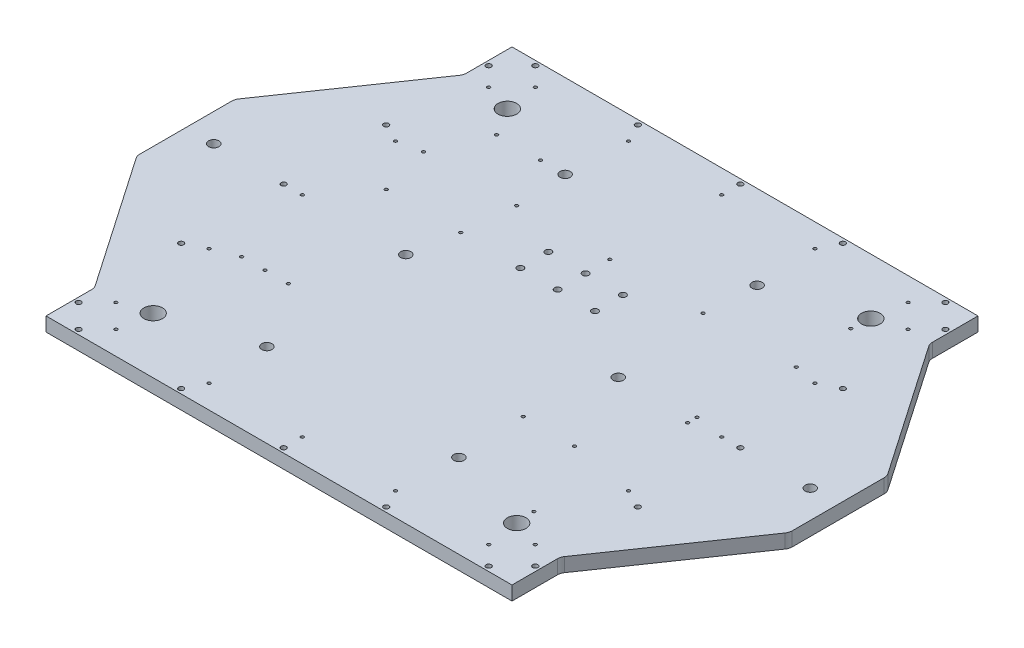
SolidWorks part; units mm, degrees
material "6061Al"
ref_plane "前视基准面" through (0, 0, 0) normal (0, 0, 1) x (1, 0, 0)
ref_plane "上视基准面" through (0, 0, 0) normal (0, 1, 0) x (1, 0, 0)
ref_plane "右视基准面" through (0, 0, 0) normal (1, 0, 0) x (0, 0, -1)
sketch "草图1" plane through (0, 0, 0) normal (0, 1, 0) x (1, 0, 0)
  line L1 (-350, -250) -> (350, -250)
  line L2 (-350, -250) -> (-350, 250)
  line L3 (-350, 250) -> (350, 250)
  line L4 (350, -250) -> (350, 250)
  line L5 (-350, -250) -> (350, 250) construction
  line L6 (-350, 250) -> (350, -250) construction
  point P0 (0, 0)
  dimension "D1" = 700
  dimension "D2" = 500
extrude "凸台-拉伸1" add sketch "草图1" along normal blind 15
sketch "草图2" plane through (0, 15, 0) normal (0, 1, 0) x (1, 0, 0)
  line L0 (-250, 250) -> (-250, 198)
  line L1 (350, 250) -> (-350, 250) construction
  line L2 (-250, 198) -> (-350, 52.5)
  line L3 (-350, 250) -> (-350, 52.5)
  line L4 (-350, 250) -> (-350, -250) construction
  line L5 (-350, 0) -> (0, 0) construction
  line L6 (0, 0) -> (0, 250) construction
  line L7 (-350, 250) -> (-250, 250)
  line L8 (350, 250) -> (250, 250)
  line L9 (350, 250) -> (350, 52.5)
  line L10 (250, 198) -> (350, 52.5)
  line L11 (250, 250) -> (250, 198)
  line L12 (250, -250) -> (250, -198)
  line L13 (250, -198) -> (350, -52.5)
  line L14 (350, -250) -> (350, -52.5)
  line L15 (350, -250) -> (250, -250)
  line L16 (-350, -250) -> (-250, -250)
  line L17 (-350, -250) -> (-350, -52.5)
  line L18 (-250, -198) -> (-350, -52.5)
  line L19 (-250, -250) -> (-250, -198)
  dimension "D1" = 52
  dimension "D2" = 100
  dimension "D3" = 105
extrude "切除-拉伸1" cut sketch "草图2" against normal through all
hole_wizard "M5 六角凹头螺钉的柱形沉头孔2" positions "草图3" profile "草图4" counterbore size "M5" standard "ISO" end condition through all
sketch "草图3" plane through (0, 0, 0) normal (0, -1, 0) x (-1, 0, 0)
  line L0 (0, 0) -> (0, 372.2873) construction
  line L2 (0, 0) -> (463.0821, 0) construction
  point P0 (-220, 245)
  point P3 (-110, 245)
  point P6 (-110, 245)
  point P8 (0, 245)
  point P11 (110, 245)
  point P14 (220, 245)
  point P17 (245, 220)
  point P20 (245, 110)
  point P33 (245, 0)
  point P37 (245, -110)
  point P38 (245, -220)
  point P39 (220, -245)
  point P40 (110, -245)
  point P41 (0, -245)
  point P42 (-110, -245)
  point P43 (-220, -245)
  point P44 (-245, -220)
  point P45 (-245, -110)
  point P46 (-245, 0)
  point P47 (-245, 110)
  point P48 (-245, 220)
sketch "草图4" plane through (220, 0, -245) normal (1, 0, 0) x (0, 0, -1)
  line L0 (0, 0) -> (0, 15)
  line L1 (0, 15) -> (2.75, 15)
  line L3 (2.75, 15) -> (2.75, 5.4)
  line L4 (2.75, 5.4) -> (4.95, 5.4)
  line L5 (4.95, 5.4) -> (4.95, 0)
  line L7 (4.95, 0) -> (0, 0)
  line L11 (0, -6.35) -> (0, 107.95) construction
  dimension "通孔孔直径" = 5.5
  dimension "通孔孔深度" = 15
  dimension "柱形沉头孔直径" = 9.9
  dimension "柱形沉头孔深度" = 5.4
hole_wizard "M10 间隙孔1" positions "草图5" profile "草图6" hole size "M10" standard "ISO" end condition through all
sketch "草图5" plane through (0, 0, 0) normal (0, -1, 0) x (-1, 0, 0)
  line L0 (0, 0) -> (0, 300.0763) construction
  line L2 (-350, -52.5) -> (-350, 52.5) construction
  line L3 (0, 0) -> (425.5875, 0) construction
  point P0 (-320, 0)
  point P2 (-114, 0)
  point P13 (114, 0)
  point P14 (320, 0)
  point P15 (-103, 160)
  point P18 (103, 160)
  point P27 (103, -160)
  point P28 (-103, -160)
  dimension "D1" = 206
  dimension "D2" = 30
sketch "草图6" plane through (320, 0, 0) normal (1, 0, 0) x (0, 0, -1)
  line L0 (0, 0) -> (0, 15)
  line L1 (0, 15) -> (5.5, 15)
  line L2 (5.5, 15) -> (5.5, 0)
  line L5 (5.5, 0) -> (0, 0)
  line L11 (0, -6.35) -> (0, 107.95) construction
  dimension "通孔孔直径" = 11
  dimension "通孔孔深度" = 15
sketch "草图9" plane through (0, 0, 0) normal (0, -1, 0) x (1, 0, 0)
  line L1 (-195, 190) -> (195, 190) construction
  line L2 (-195, 190) -> (-195, -190) construction
  line L3 (-195, -190) -> (195, -190) construction
  line L4 (195, 190) -> (195, -190) construction
  line L5 (-195, 190) -> (195, -190) construction
  line L6 (-195, -190) -> (195, 190) construction
  circle A1 centre (195, 190) radius 10
  circle A2 centre (195, -190) radius 10
  circle A3 centre (-195, -190) radius 10
  circle A4 centre (-195, 190) radius 10
  point P0 (0, 0)
  dimension "D1" = 20
  dimension "D2" = 380
  dimension "D3" = 390
extrude "切除-拉伸2" cut sketch "草图9" against normal through all
hole_wizard "M8 螺纹孔2" positions "草图10" profile "草图11" tap size "M8" standard "ISO" end condition up to next
sketch "草图10" plane through (0, 15, 0) normal (0, 1, 0) x (1, 0, 0)
  point P0 (-40, 79)
  point P3 (0, 79)
  point P6 (40, 79)
  point P9 (40, 49)
  point P12 (0, 49)
  point P15 (-40, 49)
sketch "草图11" plane through (-40, 15, -79) normal (1, 0, 0) x (0, 0, 1)
  line L0 (0, 0) -> (0, 15)
  line L1 (0, 15) -> (3.4, 15)
  line L2 (3.4, 15) -> (3.4, 0)
  line L5 (3.4, 0) -> (0, 0)
  line L11 (0, -6.35) -> (0, 107.95) construction
  dimension "通孔螺纹孔钻头直径" = 6.8
  dimension "通孔螺纹孔钻头深度" = 15
cosmetic thread "孔螺蚊线7" parameters "D2"=8
cosmetic thread "孔螺蚊线8" parameters "D2"=8
cosmetic thread "孔螺蚊线9" parameters "D2"=8
cosmetic thread "孔螺蚊线10" parameters "D2"=8
cosmetic thread "孔螺蚊线11" parameters "D2"=8
cosmetic thread "孔螺蚊线12" parameters "D2"=8
hole_wizard "M4 螺纹孔1" positions "草图12" profile "草图13" tap size "M4" standard "ISO" end condition through all
sketch "草图12" plane through (0, 15, 0) normal (0, 1, 0) x (1, 0, 0)
  line L0 (0, 250) -> (0, 0) construction
  line L1 (250, 250) -> (-250, 250) construction
  line L3 (0, 225) -> (100, 225) construction
  line L4 (0, 0) -> (381.3824, 0) construction
  line L5 (250, -198) -> (250, -250) construction
  line L6 (225, 0) -> (225, 100) construction
  line L7 (-225, 0) -> (-225, 100) construction
  line L8 (0, -225) -> (100, -225) construction
  line L9 (0, 105) -> (100, 105) construction
  line L10 (-100, 225) -> (-100, 105) construction
  point P0 (0, 225)
  point P12 (100, 225)
  point P13 (200, 225)
  point P16 (-200, 225)
  point P17 (-100, 225)
  point P23 (225, 0)
  point P32 (225, 100)
  point P33 (225, 200)
  point P36 (225, -200)
  point P37 (225, -100)
  point P40 (-225, -100)
  point P41 (-225, -200)
  point P42 (-225, 200)
  point P43 (-225, 100)
  point P44 (-225, 0)
  point P47 (-100, -225)
  point P48 (-200, -225)
  point P49 (200, -225)
  point P50 (100, -225)
  point P51 (0, -225)
  point P56 (0, 105)
  point P57 (100, 105)
  point P58 (200, 105)
  point P61 (-200, 105)
  point P62 (-100, 105)
  dimension "D1" = 25
  dimension "D3" = 100
  dimension "D4" = 25
  dimension "D6" = 100
  dimension "D8" = 120
  dimension "D2" = 3
  dimension "D5" = 3
  dimension "D7" = 2
sketch "草图13" plane through (0, 15, -225) normal (1, 0, 0) x (0, 0, 1)
  line L0 (0, 0) -> (0, 15)
  line L1 (0, 15) -> (1.65, 15)
  line L2 (1.65, 15) -> (1.65, 0)
  line L5 (1.65, 0) -> (0, 0)
  line L11 (0, -6.35) -> (0, 107.95) construction
  dimension "通孔螺纹孔钻头直径" = 3.3
  dimension "通孔螺纹孔钻头深度" = 15
cosmetic thread "孔螺蚊线13" parameters "D2"=4
cosmetic thread "孔螺蚊线14" parameters "D2"=4
cosmetic thread "孔螺蚊线15" parameters "D2"=4
cosmetic thread "孔螺蚊线16" parameters "D2"=4
cosmetic thread "孔螺蚊线17" parameters "D2"=4
cosmetic thread "孔螺蚊线18" parameters "D2"=4
cosmetic thread "孔螺蚊线19" parameters "D2"=4
cosmetic thread "孔螺蚊线20" parameters "D2"=4
cosmetic thread "孔螺蚊线21" parameters "D2"=4
cosmetic thread "孔螺蚊线22" parameters "D2"=4
cosmetic thread "孔螺蚊线23" parameters "D2"=4
cosmetic thread "孔螺蚊线24" parameters "D2"=4
cosmetic thread "孔螺蚊线25" parameters "D2"=4
cosmetic thread "孔螺蚊线26" parameters "D2"=4
cosmetic thread "孔螺蚊线27" parameters "D2"=4
cosmetic thread "孔螺蚊线28" parameters "D2"=4
cosmetic thread "孔螺蚊线29" parameters "D2"=4
cosmetic thread "孔螺蚊线30" parameters "D2"=4
cosmetic thread "孔螺蚊线31" parameters "D2"=4
cosmetic thread "孔螺蚊线32" parameters "D2"=4
cosmetic thread "孔螺蚊线46" parameters "D2"=4
cosmetic thread "孔螺蚊线47" parameters "D2"=4
cosmetic thread "孔螺蚊线48" parameters "D2"=4
cosmetic thread "孔螺蚊线49" parameters "D2"=4
cosmetic thread "孔螺蚊线50" parameters "D2"=4
hole_wizard "M4 螺纹孔2" positions "草图14" profile "草图15" tap size "M4" standard "ISO" end condition through all
sketch "草图14" plane through (0, 15, 0) normal (0, 1, 0) x (1, 0, 0)
  line L0 (-350, 52.5) -> (-350, -52.5) construction
  point P0 (-185, 50)
  point P3 (-105, 50)
  point P6 (-176.5, 160)
  point P9 (-129.5, 160)
  point P12 (193.5, 170)
  point P15 (193.5, 5)
  point P18 (193.5, -5)
  point P21 (193.5, -170)
  point P24 (99.5, -87.5)
  point P27 (154.5, -87.5)
  point P31 (-150, -90)
  point P33 (-200, -90)
  point P36 (-175, -90)
  dimension "D1" = 50
  dimension "D2" = 25
  dimension "D3" = 150
  dimension "D4" = 90
sketch "草图15" plane through (-185, 15, -50) normal (1, 0, 0) x (0, 0, 1)
  line L0 (0, 0) -> (0, 15)
  line L1 (0, 15) -> (1.65, 15)
  line L2 (1.65, 15) -> (1.65, 0)
  line L5 (1.65, 0) -> (0, 0)
  line L11 (0, -6.35) -> (0, 107.95) construction
  dimension "通孔螺纹孔钻头直径" = 3.3
  dimension "通孔螺纹孔钻头深度" = 15
cosmetic thread "孔螺蚊线33" parameters "D2"=4
cosmetic thread "孔螺蚊线34" parameters "D2"=4
cosmetic thread "孔螺蚊线35" parameters "D2"=4
cosmetic thread "孔螺蚊线36" parameters "D2"=4
cosmetic thread "孔螺蚊线37" parameters "D2"=4
cosmetic thread "孔螺蚊线38" parameters "D2"=4
cosmetic thread "孔螺蚊线39" parameters "D2"=4
cosmetic thread "孔螺蚊线40" parameters "D2"=4
cosmetic thread "孔螺蚊线41" parameters "D2"=4
cosmetic thread "孔螺蚊线42" parameters "D2"=4
cosmetic thread "孔螺蚊线43" parameters "D2"=4
cosmetic thread "孔螺蚊线44" parameters "D2"=4
cosmetic thread "孔螺蚊线45" parameters "D2"=4
fillet "圆角1" radius 10 8 edges at (-350, 7.5, 52.5) (-350, 7.5, -52.5) (-250, 7.5, 198) (250, 7.5, 198) (350, 7.5, 52.5) (350, 7.5, -52.5) (250, 7.5, -198) (-250, 7.5, -198)
